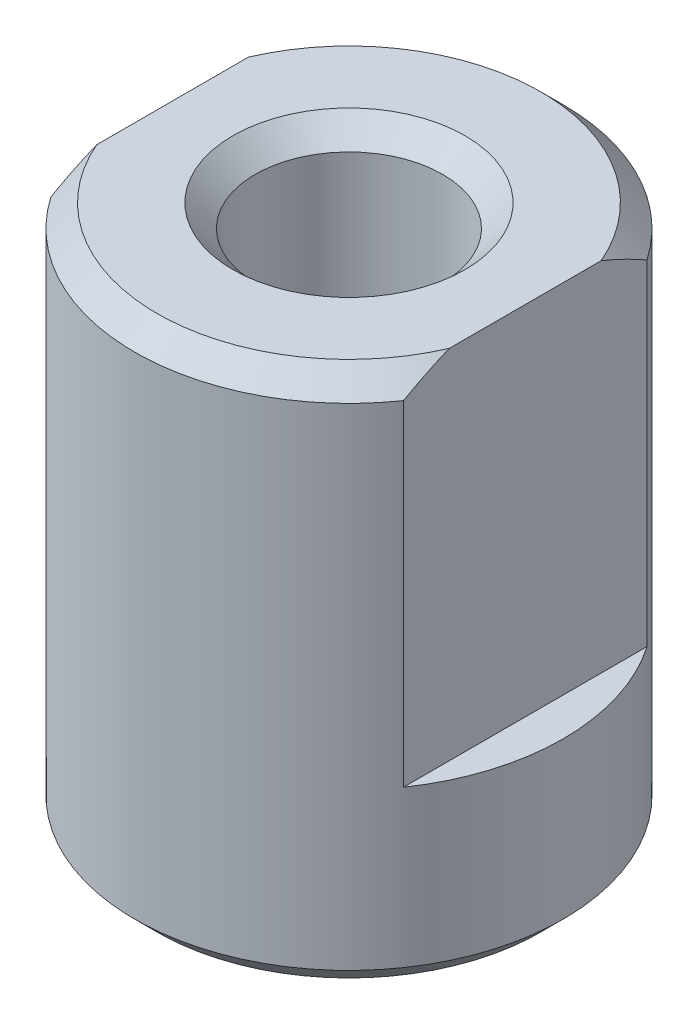
from build123d import *

# Parameters (mm, degrees)
SKETCH4_W          = 1.383873909
SKETCH4_H          = 8
CUT_EXTRUDE1_DEPTH = 5


with BuildPart() as part:
    # Sketch1 → Revolve1 (revolve)
    with BuildSketch(Plane.XY, mode=Mode.PRIVATE) as revolve1_sk:
        Polygon((0, 0), (4.3, 0), (4.8, 0.5), (4.8, 11.5), (4.3, 12), (0, 12), align=None)
    revolve(revolve1_sk.sketch.rotate(Axis((0, 12, 0), (0, 1, 0)), 90), axis=Axis((0, 12, 0), (0, 1, 0)))

    # Sketch3 → M5 Tapped Hole1 (revolve, cut)
    with BuildSketch(Plane(origin=(0, 12, 0), x_dir=(0, 0, 1), z_dir=(1, 0, 0))):
        Polygon((0, 0), (0, 12), (2.6, 12), (2.1, 11.5), (2.1, 0.5), (2.6, 0), align=None)
    revolve(axis=Axis((0, 18.35, 0), (0, -1, 0)), mode=Mode.SUBTRACT)

    # Sketch4 → Cut-Extrude1 (cut, symmetric)
    with BuildSketch(Plane.XY):
        with Locations((-4.641936955, 8)):
            Rectangle(SKETCH4_W, SKETCH4_H)
        with Locations((4.641936955, 8)):
            Rectangle(SKETCH4_W, SKETCH4_H)
    extrude(amount=CUT_EXTRUDE1_DEPTH, both=True, mode=Mode.SUBTRACT)


solid = part.part
